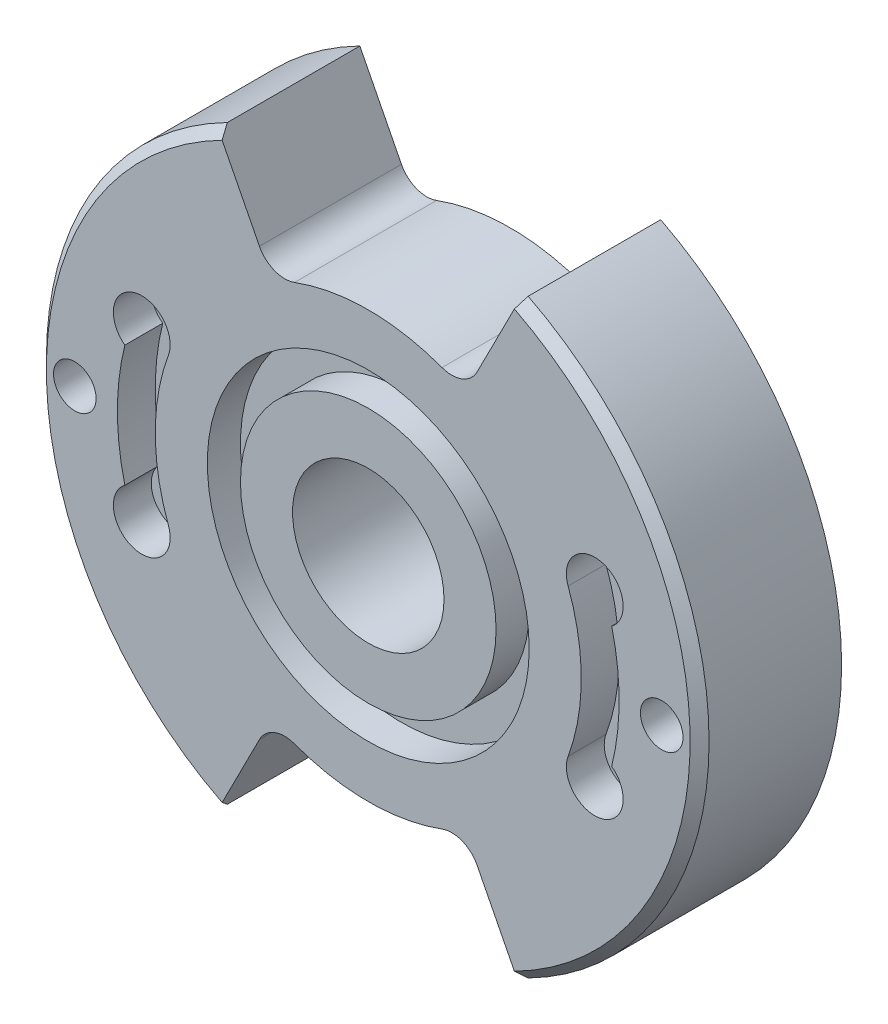
from build123d import *

# Parameters (mm, degrees)
SKETCH_1_R             = 35
EXTRUDE_1_DEPTH        = 15
CUT_EXTRUDE_1_DEPTH    = 15
FILLET_1_R             = 3
FILLET_1_OF_MIRROR_1_R = 3
SKETCH_3_R             = 17
SKETCH_3_R_2           = 13.5
CUT_EXTRUDE_2_DEPTH    = 3.5
CUT_EXTRUDE_3_DEPTH    = 4
SKETCH_5_R             = 8
CUT_EXTRUDE_4_DEPTH    = 50.21908641
SKETCH_6_R             = 2.25
CUT_EXTRUDE_5_DEPTH    = 50.21908641
CHAMFER_1_SIZE         = 1


with BuildPart() as part:
    # 草图1 → 凸台-拉伸1 (new body)
    with BuildSketch(Plane.XY):
        Circle(SKETCH_1_R)
    extrude(amount=EXTRUDE_1_DEPTH)

    # 草图2 → 切除-拉伸1 (cut)
    with BuildSketch(Plane.XY.offset(15)):
        with BuildLine():
            Line((-16.670675913, 32.718043682), (-10.214786244, 20.047646794))
            ThreePointArc((-10.214786244, 20.047646794), (0, 22.5), (10.214786244, 20.047646794))
            Line((10.214786244, 20.047646794), (16.670675913, 32.718043682))
            ThreePointArc((16.670675913, 32.718043682), (0, 36.720318868), (-16.670675913, 32.718043682))
        make_face()
    cut_extrude_1 = extrude(amount=-CUT_EXTRUDE_1_DEPTH, mode=Mode.SUBTRACT)

    # 圆角1
    fillet_1_edges = [part.edges().sort_by_distance(p)[0] for p in [
        (-10.214786244, 20.047646794, 7.5),
        (10.214786244, 20.047646794, 7.5),
    ]]
    fillet(fillet_1_edges, radius=FILLET_1_R)

    # 镜向1: 切除-拉伸1 across plane
    add(cut_extrude_1.mirror(Plane.ZX), mode=Mode.SUBTRACT)

    # 圆角1 of 镜向1
    fillet_1_of_mirror_1_edges = [part.edges().sort_by_distance(p)[0] for p in [
        (-10.214786244, -20.047646794, 7.5),
        (10.214786244, -20.047646794, 7.5),
    ]]
    fillet(fillet_1_of_mirror_1_edges, radius=FILLET_1_OF_MIRROR_1_R)

    # 草图3 → 切除-拉伸2 (cut)
    with BuildSketch(Plane.XY.offset(15)):
        Circle(SKETCH_3_R)
        Circle(SKETCH_3_R_2, mode=Mode.SUBTRACT)
    extrude(amount=-CUT_EXTRUDE_2_DEPTH, mode=Mode.SUBTRACT)

    # 草图4 → 切除-拉伸3 (cut)
    with BuildSketch(Plane.XY.offset(15)):
        with BuildLine():
            ThreePointArc((21.110164899, 7.785302689), (22.5, 0), (21.110164899, -7.785302689))
            ThreePointArc((21.110164899, -7.785302689), (24.781668408, -11.69838536), (25.712111329, -6.413839024))
            ThreePointArc((25.712111329, -6.413839024), (26.5, 0), (25.712111329, 6.413839024))
            ThreePointArc((25.712111329, 6.413839024), (24.781668408, 11.69838536), (21.110164899, 7.785302689))
        make_face()
    cut_extrude_3 = extrude(amount=-CUT_EXTRUDE_3_DEPTH, mode=Mode.SUBTRACT)

    # 镜向2: 切除-拉伸3 across plane
    add(cut_extrude_3.mirror(Plane(origin=(0, 0, 0), x_dir=(0, 0, 1), z_dir=(1, 0, 0))), mode=Mode.SUBTRACT)

    # 草图5 → 切除-拉伸4 (cut, through all)
    with BuildSketch(Plane.XY.offset(15)):
        Circle(SKETCH_5_R)
    extrude(amount=-CUT_EXTRUDE_4_DEPTH, mode=Mode.SUBTRACT)

    # 草图6 → 切除-拉伸5 (cut, through all)
    with BuildSketch(Plane.XY.offset(15)):
        with Locations((-31, 0)):
            Circle(SKETCH_6_R)
        with Locations((31, 0)):
            Circle(SKETCH_6_R)
    extrude(amount=-CUT_EXTRUDE_5_DEPTH, mode=Mode.SUBTRACT)

    # 倒角1
    chamfer_1_edges = [part.edges().sort_by_distance(p)[0] for p in [
        (35, 0, 15),
        (-35, 0, 15),
    ]]
    chamfer(chamfer_1_edges, length=CHAMFER_1_SIZE)


solid = part.part
